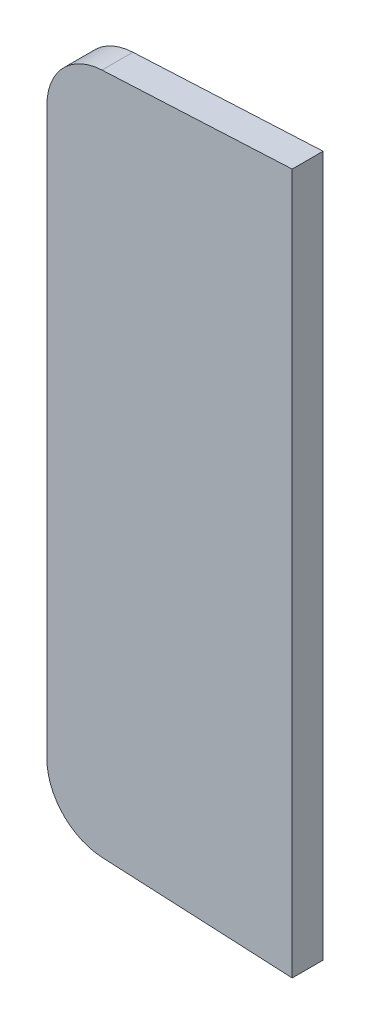
from build123d import *

# Parameters (mm, degrees)
BOSS_EXTRUDE1_DEPTH = 4


with BuildPart() as part:
    # Sketch1 → Boss-Extrude1 (new, symmetric)
    with BuildSketch(Plane.XY):
        with BuildLine():
            Line((-31.75, 73.26818434), (-31.75, -73.26818434))
            ThreePointArc((-31.75, -73.26818434), (-27.614383176, -83.610581461), (-17.487976239, -88.250019711))
            Line((-17.487976239, -88.250019711), (31.75, -90.675387205))
            Line((31.75, -90.675387205), (31.75, 90.675387205))
            Line((31.75, 90.675387205), (-17.487976239, 88.250019711))
            ThreePointArc((-17.487976239, 88.250019711), (-27.614383176, 83.610581461), (-31.75, 73.26818434))
        make_face()
    extrude(amount=BOSS_EXTRUDE1_DEPTH, both=True)


solid = part.part
